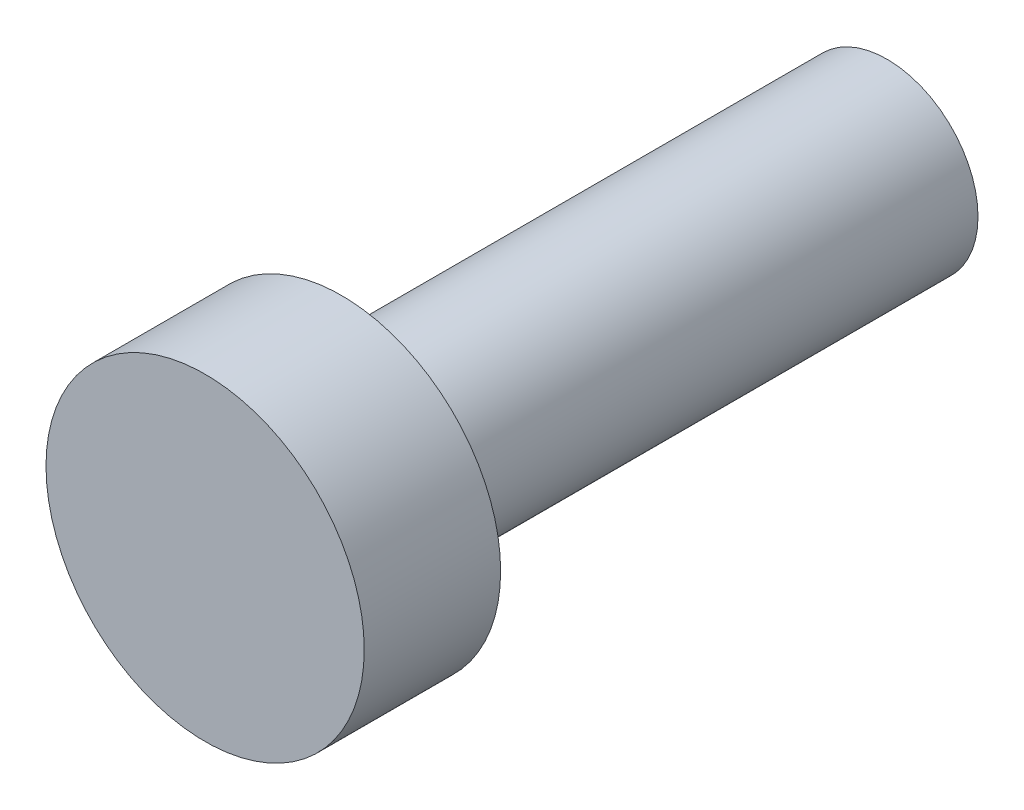
SolidWorks part; units mm, degrees
ref_plane "前视基准面" through (0, 0, 0) normal (0, 0, 1) x (1, 0, 0)
ref_plane "上视基准面" through (0, 0, 0) normal (0, 1, 0) x (1, 0, 0)
ref_plane "右视基准面" through (0, 0, 0) normal (1, 0, 0) x (0, 0, -1)
other "Configuration Table"
sketch "草图1" plane through (0, 0, 0) normal (0, 0, 1) x (1, 0, 0)
  circle A0 centre (0, 0) radius 2
  point P0 (0, 0)
  dimension "D1" = 4
extrude "凸台-拉伸1" add sketch "草图1" against normal blind 12
sketch "草图2" plane through (0, 0, 0) normal (0, 0, 1) x (1, 0, 0)
  circle A0 centre (0, 0) radius 3.5
  point P0 (0, 0)
  dimension "D1" = 7
extrude "凸台-拉伸2" add sketch "草图2" along normal blind 3
